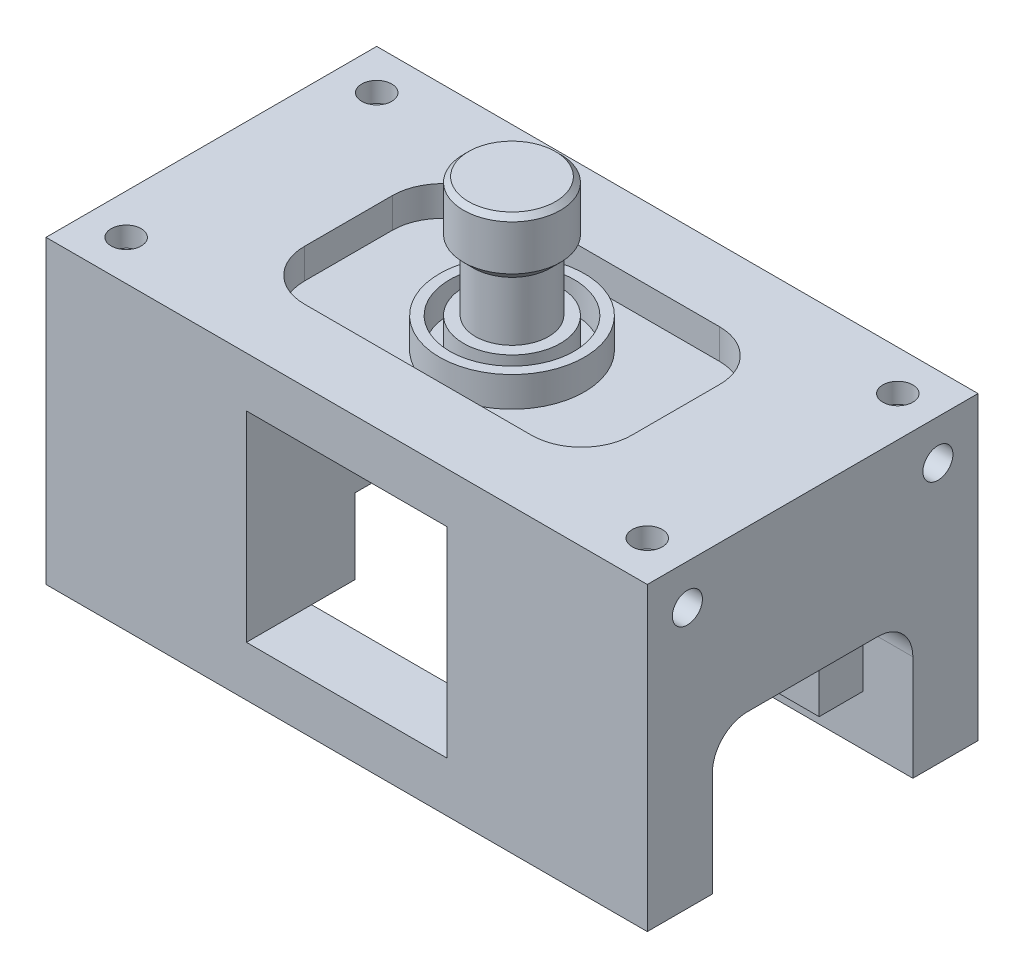
SolidWorks part; units mm, degrees
ref_plane "Front Plane" through (0, 0, 0) normal (0, 0, 1) x (1, 0, 0)
ref_plane "Top Plane" through (0, 0, 0) normal (0, 1, 0) x (1, 0, 0)
ref_plane "Right Plane" through (0, 0, 0) normal (1, 0, 0) x (0, 0, -1)
other "Configuration Table"
sketch "Sketch1" plane through (0, 0, 0) normal (0, 1, 0) x (1, 0, 0)
  line L1 (-60, 33) -> (60, 33)
  line L2 (-60, 33) -> (-60, -33)
  line L3 (-60, -33) -> (60, -33)
  line L4 (60, 33) -> (60, -33)
  line L5 (-60, 33) -> (60, -33) construction
  line L6 (-60, -33) -> (60, 33) construction
  point P0 (0, 0)
  dimension "D1" = 120
  dimension "D2" = 66
extrude "Boss-Extrude1" add sketch "Sketch1" along normal blind 60
sketch "Sketch3" plane through (60, 0, 0) normal (1, 0, 0) x (0, 0, -1)
  line L1 (-20, 10) -> (20, 10)
  line L2 (-20, 10) -> (-20, -10)
  line L3 (-20, -10) -> (20, -10)
  line L4 (20, 10) -> (20, -10)
  line L5 (-20, 10) -> (20, -10) construction
  line L6 (-20, -10) -> (20, 10) construction
  point P0 (0, 0)
  dimension "D1" = 40
  dimension "D2" = 20
extrude "Cut-Extrude1" cut sketch "Sketch3" against normal blind 120
sketch "Sketch4" plane through (0, 0, 33) normal (0, 0, 1) x (1, 0, 0)
  line L0 (-60, 60) -> (60, 60) construction
  line L1 (-20, 50) -> (20, 50)
  line L2 (-20, 50) -> (-20, 10)
  line L3 (-20, 10) -> (20, 10)
  line L4 (20, 50) -> (20, 10)
  line L5 (-20, 50) -> (20, 10) construction
  line L6 (-20, 10) -> (20, 50) construction
  point P0 (0, 30)
  dimension "D1" = 40
  dimension "D2" = 40
  dimension "D3" = 10
extrude "Cut-Extrude2" cut sketch "Sketch4" against normal blind 120
sketch "Sketch5" plane through (60, 0, 0) normal (1, 0, 0) x (0, 0, -1)
  line L0 (20, 10) -> (-20, 10) construction
  line L1 (-11.2996, 25) -> (11.2996, 25)
  line L2 (-11.2996, 25) -> (-11.2996, -5)
  line L3 (-11.2996, -5) -> (11.2996, -5)
  line L4 (11.2996, 25) -> (11.2996, -5)
  line L5 (-11.2996, 25) -> (11.2996, -5) construction
  line L6 (-11.2996, -5) -> (11.2996, 25) construction
  point P0 (0, 10)
  dimension "D1" = 30
extrude "Cut-Extrude3" cut sketch "Sketch5" against normal blind 120
sketch "Sketch6" plane through (60, 0, 0) normal (1, 0, 0) x (0, 0, -1)
  line L0 (-33, 60) -> (33, 60) construction
  line L1 (-33, 60) -> (-33, 0) construction
  line L2 (33, 60) -> (33, 0) construction
  circle A0 centre (-25, 52) radius 3
  circle A1 centre (25, 52) radius 3
  dimension "D1" = 6
  dimension "D2" = 6
  dimension "D3" = 8
  dimension "D4" = 8
  dimension "D5" = 8
  dimension "D6" = 8
extrude "Cut-Extrude4" cut sketch "Sketch6" against normal blind 120
sketch "Sketch7" plane through (60, 0, 0) normal (1, 0, 0) x (0, 0, -1)
  line L0 (-20, 10) -> (20, 10)
  line L1 (-20, 10) -> (-20, 28)
  line L2 (20, 10) -> (20, 28)
  line L3 (-20, 28) -> (20, 28)
  dimension "D1" = 18
extrude "Cut-Extrude5" cut sketch "Sketch7" against normal blind 10
sketch "Sketch8" plane through (-60, 0, 0) normal (-1, 0, 0) x (0, 0, 1)
  line L0 (-20, 10) -> (20, 10)
  line L1 (-20, 10) -> (-20, 28)
  line L2 (20, 10) -> (20, 28)
  line L3 (-20, 28) -> (20, 28)
  line L4 (11.2996, 10) -> (20, 10) construction
  line L5 (20, 10) -> (20, 0) construction
  dimension "D1" = 18
extrude "Cut-Extrude6" cut sketch "Sketch8" against normal blind 10
sketch "Sketch9" plane through (0, 60, 0) normal (0, 1, 0) x (1, 0, 0)
  line L1 (-32.6538, 18.7613) -> (32.6538, 18.7613)
  line L2 (-32.6538, 18.7613) -> (-32.6538, -18.7613)
  line L3 (-32.6538, -18.7613) -> (32.6538, -18.7613)
  line L4 (32.6538, 18.7613) -> (32.6538, -18.7613)
  line L5 (-32.6538, 18.7613) -> (32.6538, -18.7613) construction
  line L6 (-32.6538, -18.7613) -> (32.6538, 18.7613) construction
  point P0 (0, 0)
extrude "Cut-Extrude7" cut sketch "Sketch9" against normal blind 6
fillet "Fillet1" radius 10 4 edges at (32.6538, 57, -18.7613) (32.6538, 57, 18.7613) (-32.6538, 57, 18.7613) (-32.6538, 57, -18.7613)
sketch "Sketch10" plane through (0, 60, 0) normal (0, 1, 0) x (1, 0, 0)
  line L0 (60, 33) -> (-60, 33) construction
  line L1 (-60, 33) -> (-60, -33) construction
  circle A0 centre (-52, 25) radius 3
  circle A1 centre (52, 25) radius 3
  circle A2 centre (-52, -25) radius 3
  circle A3 centre (52, -25) radius 3
  dimension "D1" = 6
  dimension "D3" = 8
  dimension "D2" = 8
  dimension "D4" = 2
  dimension "D5" = 2
extrude "Cut-Extrude8" cut sketch "Sketch10" against normal blind 4
fillet "Fillet2" radius 7 4 edges at (55, 28, -20) (55, 28, 20) (-55, 28, -20) (-55, 28, 20)
sketch "Sketch11" plane through (0, 54, 0) normal (0, 1, 0) x (1, 0, 0)
  circle A0 centre (0, 0) radius 14.4571
  circle A1 centre (0, 0) radius 12.4077
extrude "Boss-Extrude2" add sketch "Sketch11" along normal blind 6
sketch "Sketch12" plane through (0, 54, 0) normal (0, 1, 0) x (1, 0, 0)
  circle A0 centre (0, 0) radius 9.6678
extrude "Boss-Extrude3" add sketch "Sketch12" along normal blind 6
sketch "Sketch13" plane through (0, 60, 0) normal (0, 1, 0) x (1, 0, 0)
  circle A0 centre (0, 0) radius 7.3107
extrude "Boss-Extrude4" add sketch "Sketch13" along normal blind 12
sketch "Sketch14" plane through (0, 72, 0) normal (0, 1, 0) x (1, 0, 0)
  circle A0 centre (0, 0) radius 9.6678
extrude "Boss-Extrude5" add sketch "Sketch14" along normal blind 12
chamfer "Chamfer1" distance 2 angle 45 1 edges at (0, 72, 9.6678)
chamfer "Chamfer2" distance 1 angle 45 1 edges at (0, 84, 9.6678)
